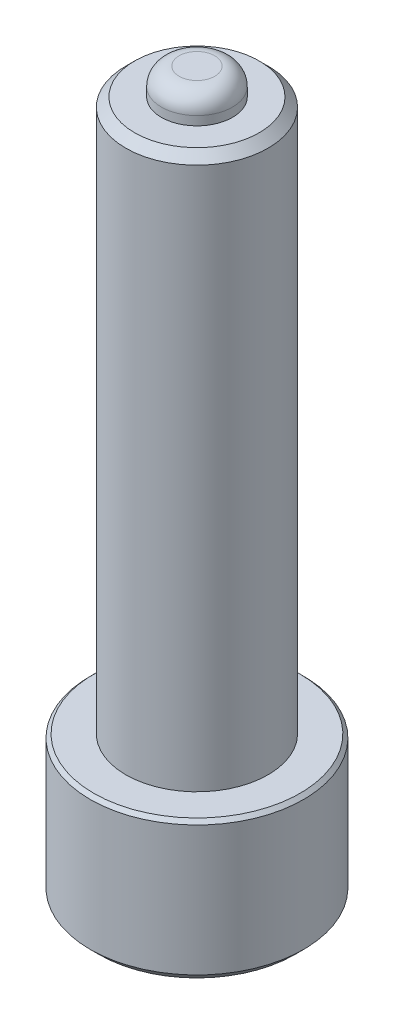
SolidWorks part; units mm, degrees
material "45"
ref_plane "Front Plane" through (0, 0, 0) normal (0, 0, 1) x (1, 0, 0)
ref_plane "Top Plane" through (0, 0, 0) normal (0, 1, 0) x (1, 0, 0)
ref_plane "Right Plane" through (0, 0, 0) normal (1, 0, 0) x (0, 0, -1)
sketch "Sketch1" plane through (0, 0, 0) normal (0, 1, 0) x (1, 0, 0)
  circle A0 centre (0, 0) radius 6
  dimension "D1" = 12
extrude "Boss-Extrude1" add sketch "Sketch1" along normal mid plane 8
sketch "Sketch2" plane through (0, 4, 0) normal (0, 1, 0) x (1, 0, 0)
  circle A0 centre (0, 0) radius 4
  dimension "D1" = 8
extrude "Boss-Extrude2" add sketch "Sketch2" along normal blind 31
cosmetic thread "Cosmetic Thread3" parameters "D1"=30, "D2"=6.647
sketch "Sketch3" plane through (0, 35, 0) normal (0, 1, 0) x (1, 0, 0)
  circle A0 centre (0, 0) radius 2
  dimension "D1" = 4
extrude "Boss-Extrude3" add sketch "Sketch3" along normal blind 1.5
sketch "Sketch4" plane through (0, -4, 0) normal (0, -1, 0) x (1, 0, 0)
  line L1 (2.8868, 0) -> (1.4434, 2.5)
  line L2 (1.4434, 2.5) -> (-1.4434, 2.5)
  line L3 (-1.4434, 2.5) -> (-2.8868, 0)
  line L4 (-2.8868, 0) -> (-1.4434, -2.5)
  line L5 (-1.4434, -2.5) -> (1.4434, -2.5)
  line L6 (1.4434, -2.5) -> (2.8868, 0)
  circle A0 centre (0, 0) radius 2.5 construction
  dimension "D1" = 5
extrude "Cut-Extrude1" cut sketch "Sketch4" against normal blind 4
chamfer "Chamfer1" distance 0.5 angle 45 2 edges at (0, 35, 4) (0, -4, 6)
chamfer "Chamfer2" distance 0.2 angle 45 1 edges at (0, 4, 6)
fillet "Fillet1" radius 1 1 edges at (0, 36.5, 2)
sketch "Sketch5" plane through (0, 0, 0) normal (1, 0, 0) x (0, 0, -1)
  line L0 (0, 0) -> (0, -7.9254) construction
  line L1 (2.5, 0) -> (0, 1.4434)
  line L2 (0, 1.4434) -> (0, 0)
  line L3 (0, 0) -> (2.5, 0)
  dimension "D1" = 60
revolve "Cut-Revolve1" cut sketch "Sketch5" angle 360 about L0
sketch "Sketch6" plane through (0, 0, 0) normal (0, 0, 1) x (1, 0, 0)
  line L0 (-5.5, -4) -> (5.5, -4) construction
  line L1 (0, 4) -> (0, -5.7899) construction
  line L2 (5.8, 4) -> (-5.8, 4) construction
  circle A0 centre (0, -0.5) radius 1.75
  dimension "D1" = 3.5
  dimension "D2" = 3.5
extrude "Cut-Extrude2" [suppressed] cut sketch "Sketch6" against normal mid plane 19
pattern_circular "CirPattern1" [suppressed] count 2 every 90
